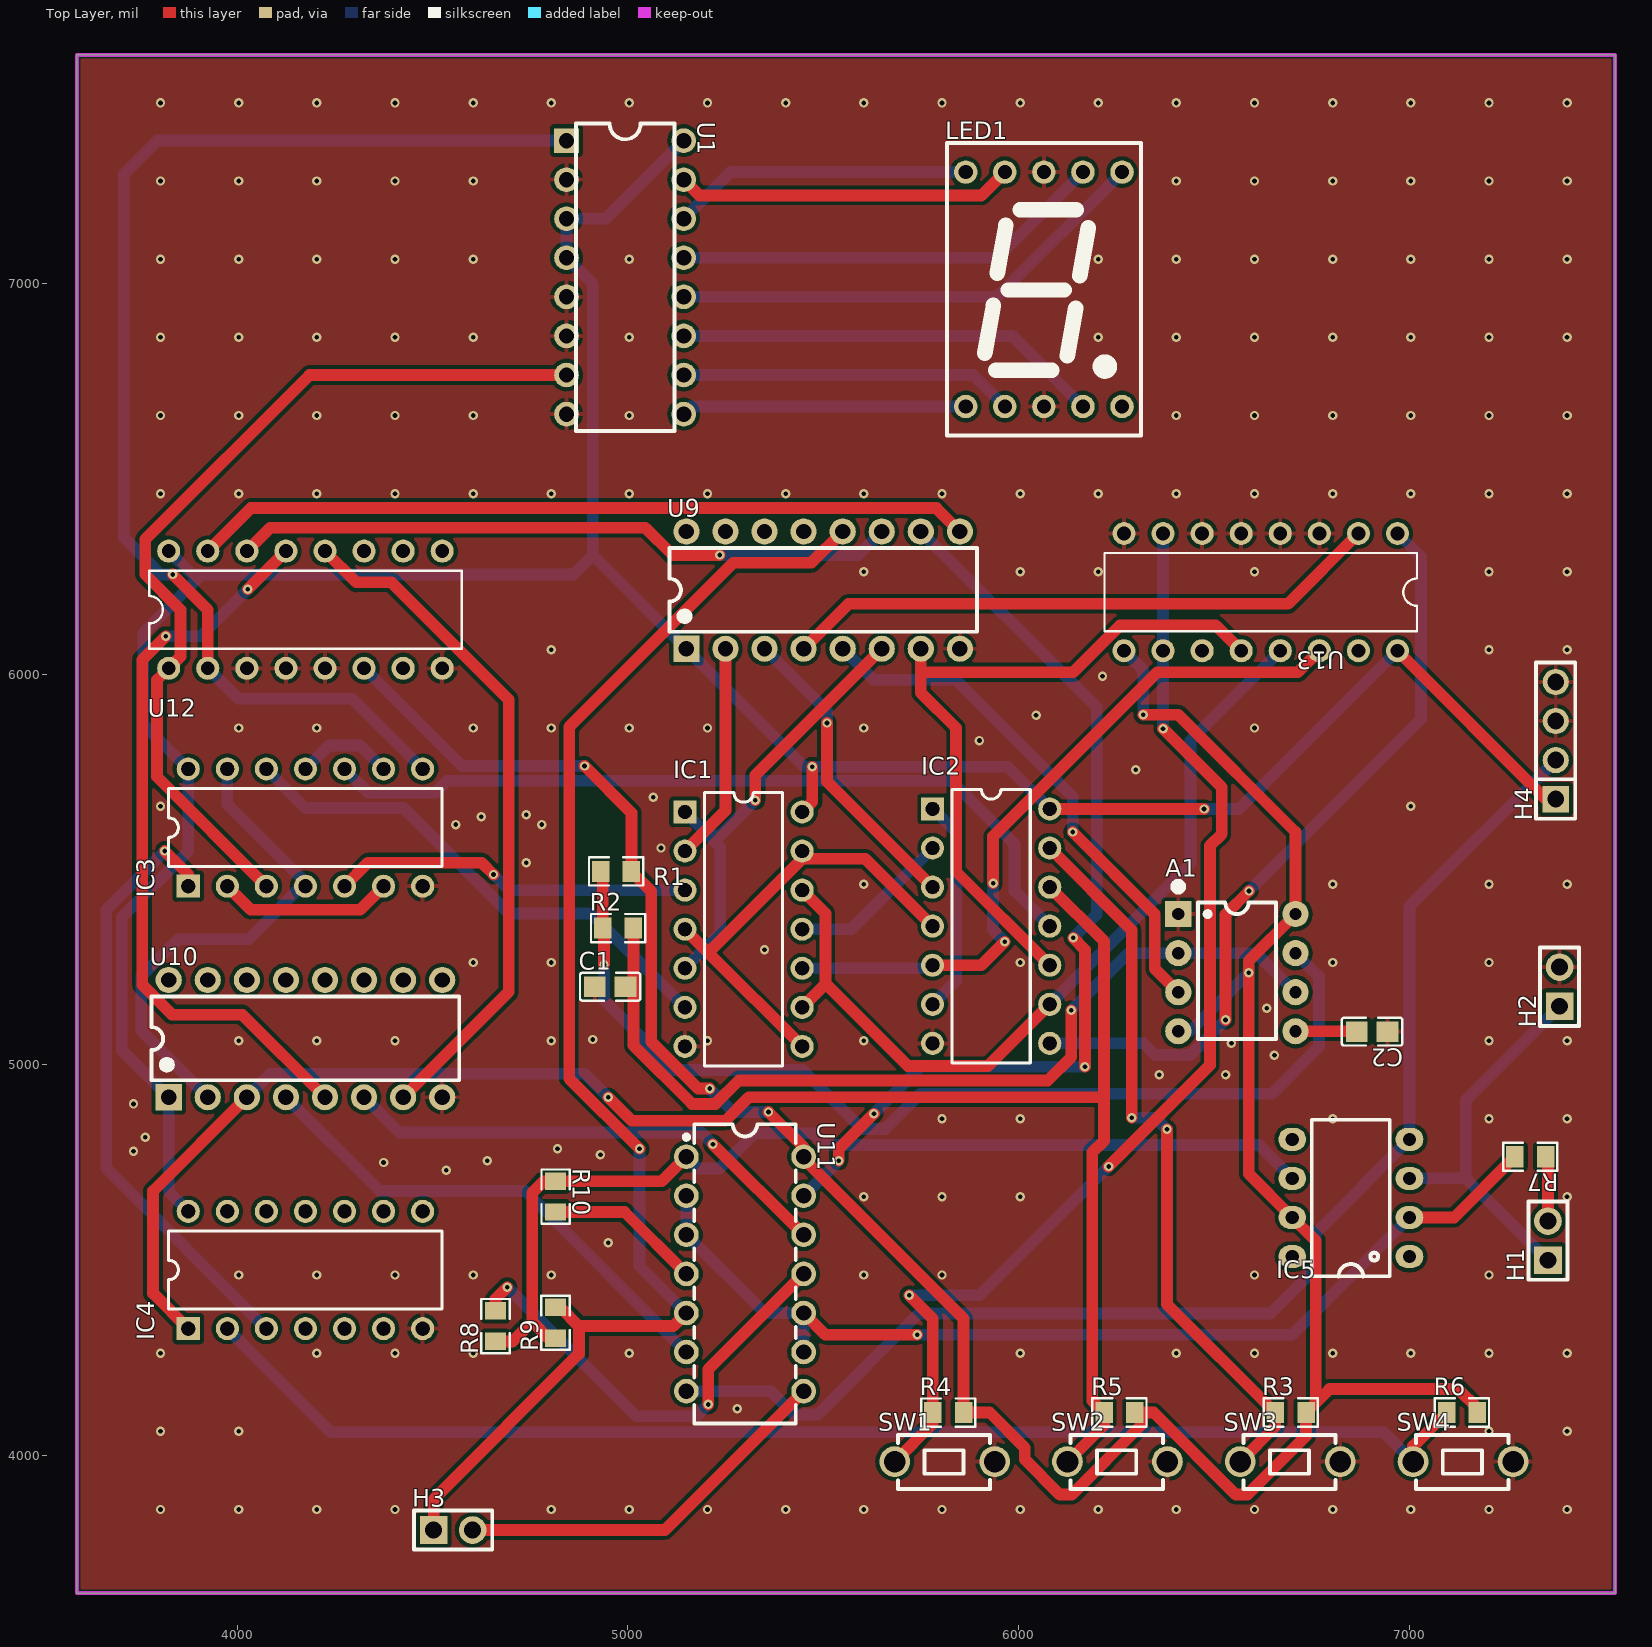
[diagram p0: Top Layer view]
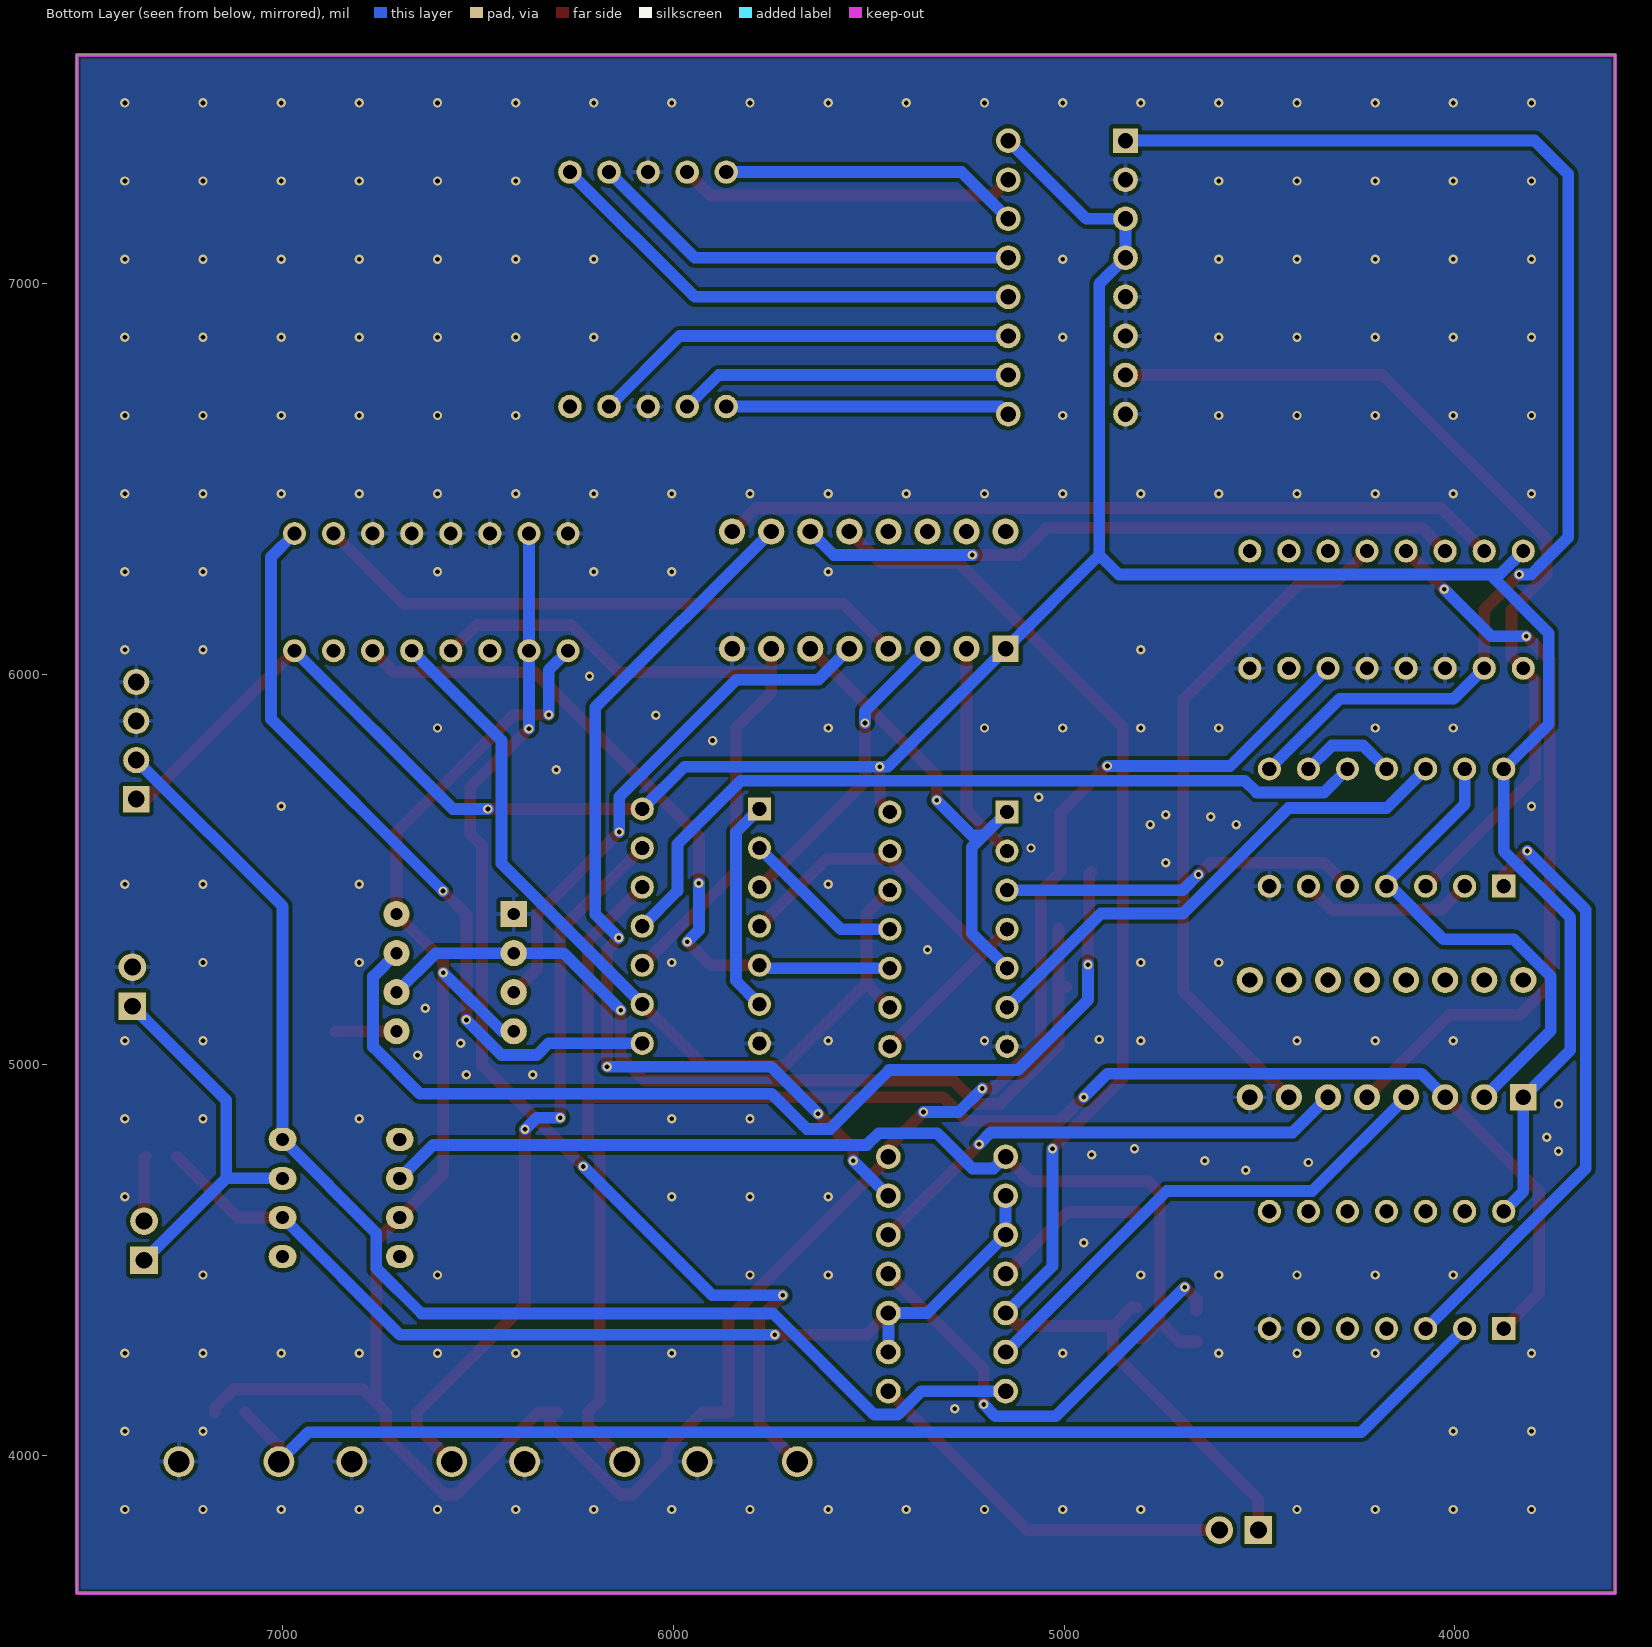
[diagram p1: Bottom Layer view, seen from below]
# Altium PCB MISC51042.pcbdoc
Units mil, origin at the board's own origin, x right, y up, seen from the top; angles counter-clockwise.
Board outline 3937.01 x 3937.01 mil, 2 copper layers (Top Layer, Bottom Layer), stack 62.206 mil thick; 33 components, 54 nets, 218 pads, 240 vias.

## Layer stack, top to bottom
Top Solder Mask Layer: solder mask 0.394, Dk 3.3
Top Layer: signal copper 1.379
Dielectric1: surface 59.449, FR4, Dk 4.5
Bottom Layer: signal copper 1.378
Bottom Solder Mask Layer: solder mask 0.394, Dk 3.3

## Board outline
3590,7585 3590,3647.99 7527.01,3647.99 7527.01,7585

## Design rules (kind name [scope] priority, off if disabled: settings)
BoardOutlineClearance copperThickness2oz_1 [All] p2 off: genericclearance=7.99 ignorepadtopadclearanceinfootprint=FALSE except(0: Arc-SplitContinuation Track-SplitContinuation SMDPad-SplitContinuation THPad-SplitContinuation Via-SplitContinuation Fill-SplitContinuation Region-SplitContinuation Poly-SplitContinuation Text-SplitContinuation Hole-SplitContinuation; 5.98: Arc-CutoutEdge SMDPad-CutoutEdge THPad-CutoutEdge Via-CutoutEdge Fill-CutoutEdge Region-CutoutEdge Text-CutoutEdge; 6.93: Hole-OutlineEdge Hole-CutoutEdge; 10: Poly-OutlineEdge Poly-CutoutEdge; 11.81: Arc-OutlineEdge Track-OutlineEdge SMDPad-OutlineEdge THPad-OutlineEdge Via-OutlineEdge Fill-OutlineEdge Region-OutlineEdge Text-OutlineEdge Track-CutoutEdge)
BoardOutlineClearance copperThickness1oz_1 [All] p4: genericclearance=4.02 ignorepadtopadclearanceinfootprint=FALSE except(0: Arc-SplitContinuation Track-SplitContinuation SMDPad-SplitContinuation THPad-SplitContinuation Via-SplitContinuation Fill-SplitContinuation Region-SplitContinuation Poly-SplitContinuation Text-SplitContinuation Hole-SplitContinuation; 6: SMDPad-CutoutEdge THPad-CutoutEdge Via-CutoutEdge Fill-CutoutEdge Region-CutoutEdge Text-CutoutEdge; 6.93: Hole-OutlineEdge Hole-CutoutEdge; 10: Poly-OutlineEdge Poly-CutoutEdge; 11.8: Arc-OutlineEdge Track-OutlineEdge SMDPad-OutlineEdge THPad-OutlineEdge Via-OutlineEdge Fill-OutlineEdge Region-OutlineEdge Text-OutlineEdge; 11.81: Arc-CutoutEdge Track-CutoutEdge)
Clearance copperThickness2oz [All] p1 off: gap=7.99 ignorepadtopadclearanceinfootprint=FALSE except(5.98: SMDPad-Track SMDPad-SMDPad THPad-Track SMDPad-THPad THPad-THPad Track-Via SMDPad-Via THPad-Via Via-Via Fill-Track Region-Track Fill-SMDPad Region-SMDPad Fill-THPad Region-THPad Fill-Via Region-Via Fill-Fill Fill-Region Region-Region Arc-Track Arc-SMDPad Arc-THPad Arc-Via Fill-Arc Region-Arc Arc-Arc Text-Track SMDPad-Text Text-THPad Text-Via Fill-Text Region-Text Arc-Text Text-Text; 6.93: Hole-Track Hole-SMDPad Hole-THPad Hole-Via Fill-Hole Region-Hole Hole-Arc Hole-Text; 10: Poly-Track Poly-SMDPad Poly-THPad Poly-Via Poly-Fill Poly-Region Poly-Poly Poly-Arc Poly-Text Poly-Hole)
Clearance copperThickness1oz [All] p3: gap=4.02 ignorepadtopadclearanceinfootprint=FALSE except(5.98: SMDPad-Track SMDPad-SMDPad THPad-Track SMDPad-THPad THPad-THPad Track-Via SMDPad-Via THPad-Via Via-Via Fill-Track Region-Track Fill-SMDPad Region-SMDPad Fill-THPad Region-THPad Fill-Via Region-Via Fill-Fill Fill-Region Region-Region; 6: Arc-Track Arc-SMDPad Arc-THPad Arc-Via Fill-Arc Region-Arc Arc-Arc Text-Track SMDPad-Text Text-THPad Text-Via Fill-Text Region-Text Arc-Text Text-Text; 6.93: Hole-Track Hole-SMDPad Hole-THPad Hole-Via Fill-Hole Region-Hole Hole-Arc Hole-Text; 10: Poly-Track Poly-SMDPad Poly-THPad Poly-Via Poly-Fill Poly-Region Poly-Poly Poly-Arc Poly-Text Poly-Hole)
Creepage creepage [All] p1: checkdistance=0 ignoreinternallayers=TRUE applytopolygonpour=TRUE
DiffPairsRouting differentialPair [All] p1: maxlimit=6 minlimit=6 mostfreqgap=6 toplayer_minwidth=5 toplayer_prefwidth=10 toplayer_maxwidth=100 toplayer_mingap=6 toplayer_prefgap=6 toplayer_maxgap=6 bottomlayer_minwidth=5 bottomlayer_prefwidth=10 bottomlayer_maxwidth=100 bottomlayer_mingap=6 bottomlayer_prefgap=6 bottomlayer_maxgap=6 maxuncoupledlength=10
HoleToHoleClearance otherClearance [All] p1: gap=11.81 allowstackedmicrovias=TRUE
Length netLength [All] p1: minlimit=0 maxlimit=0
MatchedLengths netLengthTolerance [All] p1: tolerance=1000
PasteMaskExpansion pasteMaskExpansion [All] p1: expansion=0
PlaneConnect innerPlane [All] p1: planeconnectstyle=Relief reliefexpansion=20 reliefentries=4 reliefconductorwidth=10 reliefairgap=10
PolygonConnect copperRegion [(InNet('GND'))] p1: connectstyle=Relief reliefconductorwidth=10 reliefentries=4 polygonreliefangle="90 Angle" airgapwidth=10 via.connectstyle=Relief via.reliefconductorwidth=10 via.reliefentries=4 via.polygonreliefangle="90 Angle" via.airgapwidth=10
RoutingVias viaSize [All] p1: holewidth=12.01 width=24.02 viastyle="Through Hole" minholewidth=11.81 minwidth=19.68 maxholewidth=248.03 maxwidth=393.7
SolderMaskExpansion solderMaskExpansion [IsVia] p1: expansion=-1000 istentingtop=TRUE
SolderMaskExpansion solderMaskExpansion [All] p2: expansion=2 istentingtop=FALSE
Width copperThickness2oz_2 [All] p1 off: maxlimit=100 minlimit=8 preferedwidth=10
Width copperThickness1oz_2 [All] p2: maxlimit=10 minlimit=10 preferedwidth=10 toplayer_minwidth=30 toplayer_maxwidth=100 toplayer_prefwidth=30 bottomlayer_minwidth=30 bottomlayer_maxwidth=100 bottomlayer_prefwidth=30

## Components (designator, comment, footprint, x,y, rotation, side; value= is the part's Value field where it differs from the comment)
A1 "555_VIRTUAL" 555-VIRTUAL 6559,5235.99 r0 top
C1 "10uF" C0805 4955,5200 r0 top
C2 "10nF" C0805 6905,5085 r180 top
H1 "" HDR-TH_2P-P2.54-V-M-1 7355,4550 r90 top
H2 "" HDR-TH_2P-P2.54-V-M-1 7385,5200 r90 top
H3 "" HDR-TH_2P-P2.54-V-M-1 4553.02,3809.44 r0 top
H4 "" HDR-TH_4P-P2.54-V-M 7375,5830 r90 top
IC1 "74LS00N" DIP14-300_MH 5296.32,5347.23 r0 top
IC2 "74LS00N" DIP14-300_MH 5930,5355 r0 top
IC3 "74LS00N" DIP14-300_MH 4175,5607.3 r90 top
IC4 "74LS00N" DIP14-300_MH 4175,4475 r90 top
IC5 "UA741CP" DIP8 6850.64,4659.35 r90 top
LED1 "" LED-SEG-TH_10P-L12.6-W19.0-P2.54-S15.24-BL 6065,6985 r0 top
R1 "100K" R0805 4970,5495 r180 top
R2 "20K" R0805 4975,5350 r0 top
R3 "10K" R0805 6696.67,4110.2 r0 top
R4 "10K" R0805 5820,4110 r0 top
R5 "10K" R0805 6258.33,4110.2 r0 top
R6 "10K" R0805 7135,4110.2 r0 top
R7 "10K" R0805 7310,4765 r180 top
R8 "30K" R0805 4661.38,4331.6 r90 top
R9 "20K" R0805 4815,4340 r90 top
R10 "10K" R0805 4815.12,4662.83 r270 top
SW1 "" Key_TH_3.5x6x4.3 5804.62,3984.7 r0 top
SW2 "" Key_TH_3.5x6x4.3 6246.85,3984.7 r0 top
SW3 "" Key_TH_3.5x6x4.3 6689.07,3984.7 r0 top
SW4 "" Key_TH_3.5x6x4.3 7131.29,3984.7 r0 top
U1 "" DIP-16_L19.8-W6.5-P2.54-LS7.6-BL 4993.15,7015.63 r270 top
U9 "" PDIP-16_L19.7-W6.6-P2.54-LS7.6-BL 5500,6215 r0 top
U10 "" PDIP-16_L19.7-W6.6-P2.54-LS7.6-BL 4175,5067.13 r0 top
U11 "" PDIP-14_L19.3-W6.4-P2.54-LS7.9-BL 5300,4465 r270 top
U12 "74LS138N" DIP-16_L20.32-W6.4-P2.54-LS7.6-BL 4175,6165 r0 top
U13 "74LS161DC" DIP-16_L20.32-W6.4-P2.54-LS7.6-BL 6620,6210 r180 top

## Footprints (in the part's own frame and the unit in brackets; to place one, negate y for a bottom-side part, rotate by r counter-clockwise, add the part's x,y. Pads: shape width x height; smd on the part's side, far side on the other; paste and mask are expansions set on the pad)
555-VIRTUAL [mm]
  rect 1.7x1.7 hole 0.8: 1(-3.81,3.81)
  round 1.7 hole 0.8: 2(-3.81,1.27) 3(-3.81,-1.27) 4(-3.81,-3.81) 5(3.81,-3.81) 6(3.81,-1.27) 7(3.81,1.27) 8(3.81,3.81)
  silkscreen extent -4.06,-4.32 2.54,5.84
C0805 [mm]
  rect 1.41x1.35 smd paste-100 mask+0.051: 1(-1,0) 2(1,0)
  silkscreen extent -1.96,-0.9 1.96,0.9
DIP8 [mm]
  oval 1.5x1.8 hole 0.85 paste+0 mask+0.102: 1(-3.81,-3.81) 2(-1.27,-3.81) 3(1.27,-3.81) 4(3.81,-3.81) 5(3.81,3.81) 6(1.27,3.81) 7(-1.27,3.81) 8(-3.81,3.81)
  silkscreen extent -5.1,-2.54 5.08,2.54
DIP14-300_MH [mm]
  rect 1.5x1.5 hole 0.9 slot 0.905 at 0 deg: 1(-3.81,7.62)
  round 1.5 hole 0.9 slot 0.905 at 0 deg: 2(-3.81,5.08) 3(-3.81,2.54) 4(-3.81,0) 5(-3.81,-2.54) 6(-3.81,-5.08) 7(-3.81,-7.62) 8(3.81,-7.62) 9(3.81,-5.08) 10(3.81,-2.54) 11(3.81,0) 12(3.81,2.54) 13(3.81,5.08) 14(3.81,7.62)
  silkscreen extent -2.54,-8.89 2.54,8.89
DIP-16_L19.8-W6.5-P2.54-LS7.6-BL [mm]
  rect 1.6x1.6 hole 1: 1(-8.89,-3.81)
  round 1.6 hole 1 copper offset 0,0: 2(-6.35,-3.81) 3(-3.81,-3.81) 4(-1.27,-3.81) 5(1.27,-3.81) 6(3.81,-3.81) 7(6.35,-3.81) 8(8.89,-3.81) 9(8.89,3.81) 10(6.35,3.81) 11(3.81,3.81) 12(1.27,3.81) 13(-1.27,3.81) 14(-3.81,3.81) 15(-6.35,3.81) 16(-8.89,3.81)
  silkscreen extent -10,-3.2 10,3.2
DIP-16_L20.32-W6.4-P2.54-LS7.6-BL [mm]
  round 1.5 hole 0.9: 1(-8.89,-3.81) 2(-6.35,-3.81) 3(-3.81,-3.81) 4(-1.27,-3.81) 5(1.27,-3.81) 6(3.81,-3.81) 7(6.35,-3.81) 8(8.89,-3.81) 9(8.89,3.81) 10(6.35,3.81) 11(3.81,3.81) 12(1.27,3.81) 13(-1.27,3.81) 14(-3.81,3.81) 15(-6.35,3.81) 16(-8.89,3.81)
  silkscreen extent -10.16,-2.54 10.16,2.54
HDR-TH_2P-P2.54-V-M-1 [mm]
  rect 1.8x1.8 hole 1.1: 1(-1.27,0)
  round 1.8 hole 1.1: 2(1.27,0)
  silkscreen extent -2.54,-1.27 2.54,1.27
HDR-TH_4P-P2.54-V-M [mm]
  rect 1.7x1.7 hole 1.1: 1(-3.81,0)
  round 1.7 hole 1.1: 2(-1.27,0) 3(1.27,0) 4(3.81,0)
  silkscreen extent -5.08,-1.27 5.08,1.27
Key_TH_3.5x6x4.3 [mil]
  round 78.7 hole 55.1 paste+0 mask+2: A(-121.44,0) B(134.46,0)
  silkscreen extent -114,-70 123,68
LED-SEG-TH_10P-L12.6-W19.0-P2.54-S15.24-BL [mil]
  round 60 hole 36: 1(-200,-300) 2(-100,-300) 3(0,-300) 4(100,-300) 5(200,-300) 6(200,300) 7(100,300) 8(0,300) 9(-100,300) 10(-200,300)
  silkscreen extent -248,-374 248,374
PDIP-14_L19.3-W6.4-P2.54-LS7.9-BL [mm]
  round 1.6 hole 1: 1(-7.62,-3.81) 2(-5.08,-3.81) 3(-2.54,-3.81) 4(0,-3.81) 5(2.54,-3.81) 6(5.08,-3.81) 7(7.62,-3.81) 8(7.62,3.81) 9(5.08,3.81) 10(2.54,3.81) 11(0,3.81) 12(-2.54,3.81) 13(-5.08,3.81) 14(-7.62,3.81)
  silkscreen extent -9.73,-3.96 9.73,3.3
PDIP-16_L19.7-W6.6-P2.54-LS7.6-BL [mm]
  rect 1.7x1.7 hole 1: 1(-8.89,-3.81)
  round 1.7 hole 1: 2(-6.35,-3.81) 3(-3.81,-3.81) 4(-1.27,-3.81) 5(1.27,-3.81) 6(3.81,-3.81) 7(6.35,-3.81) 8(8.89,-3.81) 9(8.89,3.81) 10(6.35,3.81) 11(3.81,3.81) 12(1.27,3.81) 13(-1.27,3.81) 14(-3.81,3.81) 15(-6.35,3.81) 16(-8.89,3.81)
  silkscreen extent -10,-2.7 10,2.73
R0805 [mm]
  rect 1.133x1.377 smd paste-100 mask+0.051: 1(-1,0) 2(1,0)
  silkscreen extent -1.76,-0.92 1.76,0.92

## Via types
v1: diameter 24.02, hole 12, Top Layer to Bottom Layer, 240 vias

## Nets (pads, with @x,y where several pads share a name; then routed paths per layer and width w, separated by ;. In a path a pad name is that pad's centre, name@x,y a point inside that pad or via, vN(x,y) a via of type N, cw(c..) or ccw(c..) an arc to the next point about the centre after c; other vN are vias at no path point)
$1N1: LED1.7 U1.13 | length 1112.7
  Bottom Layer w30: U1.13@5143.15,7065.63 5945.63,7065.63 LED1.7
$1N2: LED1.6 U1.12 | length 1254.1
  Bottom Layer w30: U1.12@5143.15,6965.63 5945.63,6965.63 LED1.6
$1N3: LED1.4 U1.11 | length 1096.7
  Bottom Layer w30: U1.11@5143.15,6865.63 5984.36,6865.63 LED1.4
$1N4: LED1.2 U1.10 | length 855.3
  Bottom Layer w30: U1.10@5143.15,6765.63 5884.36,6765.63 LED1.2
$1N5: LED1.1 U1.9 | length 729.9
  Bottom Layer w30: U1.9@5143.15,6665.63 5162.51,6685 LED1.1
$1N6: LED1.9 U1.15 | length 863.5
  Top Layer w30: U1.15@5143.15,7265.63 5183.78,7225 5905,7225 LED1.9
$1N7: LED1.10 U1.14 | length 771.3
  Bottom Layer w30: U1.14@5143.15,7165.63 5262.51,7285 LED1.10
$1N10: IC1.2 U9.2 | length 560.7
  Top Layer w30: IC1.2 5250,5650.91 U9.2
$1N11: IC1.1 IC1.5 U9.6 | length 1153.7
  Top Layer w30: v1(5326.32,5677.23) 5326.32,5741.32 U9.6
  Bottom Layer w30: IC1.5 5236.32,5337.23 5236.32,5557.23 5206.32,5587.23 ; IC1.1 5206.32,5587.23 ; v1(5326.32,5677.23) 5236.32,5587.23 5206.32,5587.23
$1N12: IC1.6 IC3.12 | length 1324
  Bottom Layer w30: IC3.12 4175.07,5657.23 4426.32,5657.23 4696.32,5387.23 4906.32,5387.23 IC1.6
$1N13: IC1.4 IC1.8 IC1.13 IC2.4 | length 1188.7
  Top Layer w30: IC1.4 5206.32,5287.23 ; IC1.8 5206.32,5287.23 ; IC1.13 IC1.13@5446.32,5527.23 ; IC2.4 5607.77,5527.23 IC1.13@5446.32,5527.23 ; 5206.32,5287.23 IC1.13@5446.32,5527.23
$1N15: IC1.10 IC2.5 U13.14 | length 1860.9
  Top Layer w30: IC2.5 5905,5255 v1(5965,5315) ; v1(5935,5465) 5935,5585 6355,6005 6715,6005 U13.14
  Bottom Layer w30: IC1.10 5772.23,5247.23 IC2.5 ; v1(5935,5465) 5935,5345 v1(5965,5315)
$1N17: IC2.3 U9.3 | length 788.1
  Top Layer w30: v1(5510,5875) 5510,5725 IC2.3
  Bottom Layer w30: U9.3 5510,5905 v1(5510,5875)
$1N18: IC1.11 IC2.2 | length 419.7
  Bottom Layer w30: IC1.11 5572.23,5347.23 IC2.2
$1N19: IC2.1 IC2.6 | length 549.7
  Bottom Layer w30: IC2.6 5840,5215 5840,5595 IC2.1
$1N20: A1.4 A1.8 IC5.7 R1.1 R3.2 R4.2 R5.2 R6.2 U11.14 U12.6 U13.9 | length 7125.6
  Top Layer w30: v1(4889.37,5765) 5009.37,5645 R1.1 5060,5444.37 5060,5059.37 5180,4939.37 v1(5210,4939.37) ; v1(5360,4879.37) 5450,4789.37 5450,4759.37 5859.37,4350 R4.2 ; R4.2@5859.57,4110.2 5926.04,4110.2 6016.04,4020.2 6016.04,3990.2 6106.04,3900.2 6136.04,3900.2 6316.04,4080.2 R5.2@6316.04,4110.2 ; R5.2 R5.2@6316.04,4110.2 ; v1(6319,5895.99) 6409,5895.99 6709,5595.99 A1.8 6589,5265.99 v1(6589,5235.99) 6589,4721 IC5.7 6760.64,4549.35 6760.64,4134.81 ; R6.2 7174.37,4121.87 7126.04,4170.2 6796.04,4170.2 6760.64,4134.81 ; R5.2@6316.04,4110.2 6346.04,4110.2 6556.04,3900.2 6586.04,3900.2 6736.04,4050.2 R3.2 6760.64,4134.81
  Bottom Layer w30: U12.6 4575,5765 v1(4889.37,5765) ; v1(5210,4939.37) 5270,4879.37 v1(5360,4879.37) ; U13.9 6319,6011 v1(6319,5895.99) ; A1.4 6439,5085.99 v1(6589,5235.99)
$1N21: A1.7 R1.2 R2.1 | length 2650.6
  Top Layer w30: R1.2 4935.63,5490 R2.1 4939,5346.63 v1(4939,5256.63)
  Bottom Layer w30: v1(4939,5256.63) 4939,5166.63 5119,4986.63 5448.37,4986.63 5599,4836 5659,4836 5749,4926 6649,4926 6769,5045.99 6769,5225.99 A1.7
$1N22: A1.2 A1.6 C1.2 R2.2 | length 2348.4
  Top Layer w30: C1.2 C1.2@5014.37,5200 ; R2.2 C1.2@5014.37,5200 ; v1(6134.99,5140) 6134.99,5020 6074.99,4960 5284.37,4960 5224.37,4900 5164.37,4900 5014.37,5050 C1.2@5014.37,5200
  Bottom Layer w30: v1(6134.99,5140) 6280.99,5285.99 A1.2 6609,5285.99 A1.6
$1N24: A1.5 C2.2 | length 157
  Top Layer w30: A1.5 6864.63,5085.99 C2.2
$1N25: A1.3 U9.5 | length 1357.8
  Top Layer w30: v1(6139,5596) 6349,5386 6349,5245.99 A1.3
  Bottom Layer w30: U9.5 5629,5986 5839,5986 6139,5686 v1(6139,5596)
$1N26: U9.4 U13.2 | length 1542.2
  Top Layer w30: U9.4 5565,6180 6690,6180 U13.2
$1N30: R4.1 SW1.A U13.7 U13.10 | length 2939.2
  Top Layer w30: SW1.A 5780.63,4082.15 R4.1 5780.63,4350 v1(5720.63,4410) ; v1(6230.63,4740) 6490,4999.37 6490,5560.62 6520,5590.62 6520,5710.62 v1(6370,5860.62)
  Bottom Layer w30: v1(5720.63,4410) 5900.63,4410 v1(6230.63,4740) ; v1(6370,5860.62) U13.10 U13.7
$1N31: IC2.8 U13.1 | length 1976.7
  Top Layer w30: v1(6530,5115) 6530,5385 v1(6590,5445)
  Bottom Layer w30: IC2.8 6320,5055 6350,5025 6440,5025 v1(6530,5115) ; v1(6590,5445) 7030,5885 7030,6300 U13.1
$1N32: IC2.10 U9.7 U13.12 | length 1843.3
  Top Layer w30: U9.7 5750,6005 ; IC2.10 5840,5495 5840,5862.48 5750,5952.48 5750,6005 ; U13.12 6505.01,6125 6260,6125 6140,6005 5750,6005
$1N33: IC1.9 IC1.12 IC2.9 U13.13 | length 2225.1
  Top Layer w30: IC1.9 5506.32,5207.23 ; IC1.12 5506.32,5387.23 5506.32,5207.23 ; IC2.9 5922.23,4997.23 5716.32,4997.23 5506.32,5207.23
  Bottom Layer w30: IC2.9 6440,5515 6440,5830 U13.13
$1N35: IC5.6 R8.1 R9.1 R10.1 U11.1 | length 2603.1
  Top Layer w30: R8.1 4705.14,4292.22 4755.12,4342.2 ; R9.1 4796.7,4300.63 4755.12,4342.2 ; U11.1 5087.2,4702.2 R10.1 4785.12,4702.2 4755.12,4672.2 4755.12,4342.2
  Bottom Layer w30: U11.1 5180,4735 5235,4735 5325,4825 5475,4825 5505,4795 6615,4795 IC5.6
$1N36: IC5.2 R7.2 U11.2 U11.3 U11.9 U11.10 | length 2615.3
  Top Layer w30: U11.10 5505.65,4309.35 v1(5740.64,4309.35) ; IC5.2 7114.98,4609.35 R7.2
  Bottom Layer w30: U11.2 U11.3 5350,4365 U11.10 U11.9 ; v1(5740.64,4309.35) 6700.64,4309.35 IC5.2
$1N37: H1.2 R7.1 | length 167.3
  Top Layer w30: R7.1 7355,4759.37 H1.2
$1N38: H1.1 H2.1 IC5.3 | length 981
  Bottom Layer w30: IC5.3 7001.29,4710 7145,4710 ; H1.1 7145,4710 ; H2.1 7145,4910 7145,4710
$1N39: U9.9 U12.15 | length 1995.4
  Top Layer w30: U12.15 4035,6425 5790,6425 U9.9
$1N40: U9.11 U12.14 | length 1703.7
  Top Layer w30: U12.14 4085,6375 5045,6375 5115,6305 v1(5235,6305)
  Bottom Layer w30: v1(5235,6305) 5590,6305 U9.11
$1N41: U10.5 U12.13 | length 1902.2
  Top Layer w30: v1(3817.13,6097.13) 3757.13,6037.13 3757.13,5205 3833.64,5128.49 4013.64,5128.49 U10.5 ; v1(4027.13,6217.13) U12.13
  Bottom Layer w30: v1(3817.13,6097.13) 3907.13,6097.13 v1(4027.13,6217.13)
$1N42: U10.7 U12.12 | length 1757.1
  Top Layer w30: U12.12 4305,6235 4395,6235 4695,5935 4695,5187.13 U10.7
$1N43: U9.10 U11.13 | length 2467.9
  Top Layer w30: v1(5540,4755) 5540,4785 v1(5630,4875) ; v1(6140,5325) 6170,5295 v1(6170,4995)
  Bottom Layer w30: U11.13 v1(5540,4755) ; v1(5630,4875) 5750,4995 v1(6170,4995) ; U9.10 6200,5915 6200,5385 v1(6140,5325)
$1N44: H3.1 R9.2 U9.12 U11.5 | length 3576.2
  Top Layer w30: H3.1 4503.02,3888.18 4875,4260.16 4875,4331.42 ; R9.2 4827.05,4379.37 4875,4331.42 ; v1(5030,4785) 4850,4965 4850,5865 5270,6285 5470,6285 U9.12 ; U11.5 5116.42,4331.42 4875,4331.42
  Bottom Layer w30: v1(5030,4785) 5030,4485 U11.5
$1N45: U10.4 U11.6 | length 1295.1
  Bottom Layer w30: U10.4 4365,4677.13 4737.87,4677.13 U11.6
$1N46: U10.6 U11.12 | length 1270.9
  Top Layer w30: v1(5217.87,4797.13) U11.12
  Bottom Layer w30: U10.6 4415,4827.13 5187.87,4827.13 v1(5217.87,4797.13)
$1N47: R8.2 U11.11 | length 1171.2
  Top Layer w30: R8.2 4661.38,4400.96 v1(4691.38,4430.96) ; v1(5205.96,4130.97) 5205.96,4220.97 U11.11
  Bottom Layer w30: v1(4691.38,4430.96) 5021.38,4100.97 5175.96,4100.97 v1(5205.96,4130.97)
$1N48: R10.2 U11.4 | length 400.5
  Top Layer w30: R10.2 4991.54,4623.46 U11.4
$1N49: H3.2 U11.8 | length 994.3
  Top Layer w30: H3.2 5094.44,3809.44 U11.8
$1N64: IC1.3 IC3.5 | length 925.2
  Top Layer w30: IC3.5 4335,5517.3 4626.25,5517.3 v1(4656.25,5487.3)
  Bottom Layer w30: v1(4656.25,5487.3) 4696.32,5447.23 IC1.3
$1N65: IC3.4 IC3.13 U10.2 | length 1282.8
  Bottom Layer w30: U10.2 3755,5087.13 3755,5227.3 3849.32,5321.62 4029.32,5321.62 IC3.4@4175,5467.3 ; IC3.13 3975,5667.3 IC3.4@4175,5467.3 ; IC3.4 IC3.4@4175,5467.3
$1N66: IC2.12 IC4.1 R5.1 SW2.A U10.3 | length 4617.3
  Top Layer w30: IC4.1 3785,4415 3785,4677.13 U10.3 ; v1(4950.06,4917.13) 5010.06,4857.13 5250.06,4857.13 5310.06,4917.13 6210.06,4917.13 6218.96,4926.03 ; IC2.12 6218.96,5316.03 6218.96,4926.03 ; SW2.A 6218.96,4078.26 R5.1 6188.96,4140.2 6188.96,4776.03 6218.96,4806.03 6218.96,4926.03
  Bottom Layer w30: U10.3 4085,4977.13 4890.06,4977.13 v1(4950.06,4917.13)
$1N67: IC4.2 R6.1 SW4.A | length 3336.8
  Top Layer w30: SW4.A 7009.85,4024.43 R6.1
  Bottom Layer w30: IC4.2 4240,4060 6934.56,4060 SW4.A
$1N68: IC3.9 IC3.11 | length 249.7
  Bottom Layer w30: IC3.11 4235,5817.3 4315,5817.3 IC3.9
$1N69: IC2.11 IC3.10 | length 2066.8
  Bottom Layer w30: IC3.10 4335,5697.3 4507.7,5697.3 4537.7,5727.3 5827.7,5727.3 5990,5565 5990,5445 IC2.11
$1N70: IC2.13 R3.1 SW3.A | length 1881.7
  Top Layer w30: IC2.13 6290,5345 v1(6290,4865) ; v1(6380,4835) 6380,4387.5 R3.1 6657.3,4074.37 SW3.A
  Bottom Layer w30: v1(6290,4865) 6350,4865 v1(6380,4835)
$1N71: IC3.2 IC3.6 | length 449.7
  Top Layer w30: IC3.2 4035,5397.3 4315,5397.3 IC3.6
$1N72: IC3.1 IC4.3 | length 1569.1
  Top Layer w30: v1(3815,5547.3) 3875,5487.3 IC3.1
  Bottom Layer w30: v1(3815,5547.3) 3665,5397.3 3665,4735 IC4.3
$1N73: IC3.3 U1.7 U12.1 | length 2318.2
  Top Layer w30: IC3.3 3795,5737.3 3795,5985 U12.1 3855,6045 3855,6165 3765,6255 3765,6345 4185.63,6765.63 U1.7@4843.15,6765.63
$1N74: IC3.8 U1.1 U12.2 | length 3197
  Top Layer w30: v1(3835,6255) 3925,6165 U12.2
  Bottom Layer w30: v1(3835,6255) 3805,6255 3770.24,6289.76 3710,6350 3710,7280 3795.63,7365.63 U1.1 ; U12.2 4002.7,5937.3 4295,5937.3 IC3.8
GND: A1.1 C1.1 C2.1 H2.2 H4.3 H4.4 IC1.7 IC2.7 IC3.7 IC4.7 LED1.3 LED1.8 SW1.B SW2.B SW3.B SW4.B U1.2 U1.5 U1.6 U1.8 U9.8 U10.8 U12.3 U12.4 U12.5 U12.8 U13.3 U13.4 U13.5 U13.6 U13.8
  other v1: 3804.1,3862.09 4004.1,3862.09 4204.1,3862.09 4404.1,3862.09 4804.1,3862.09 5004.1,3862.09 5204.1,3862.09 5404.1,3862.09 5604.1,3862.09 5804.1,3862.09 6004.1,3862.09 6204.1,3862.09 6404.1,3862.09 6604.1,3862.09 6804.1,3862.09 7004.1,3862.09 7204.1,3862.09 7404.1,3862.09 3804.1,4062.09 4004.1,4062.09 7204.1,4062.09 7404.1,4062.09 5280,4120 3804.1,4262.09 4204.1,4262.09 4404.1,4262.09 4604.1,4262.09 5004.1,4262.09 6004.1,4262.09 6404.1,4262.09 6604.1,4262.09 6804.1,4262.09 7004.1,4262.09 7204.1,4262.09 7404.1,4262.09 4004.1,4462.09 4204.1,4462.09 4404.1,4462.09 4604.1,4462.09 4804.1,4462.09 5604.1,4462.09 5804.1,4462.09 6604.1,4462.09 7204.1,4462.09 4950,4545 5604.1,4662.09 5804.1,4662.09 6004.1,4662.09 7404.1,4662.09 4535,4730 4375,4750 4640,4755 4930,4770 3735,4778.74 4820,4785 3765,4815 5804.1,4862.09 6004.1,4862.09 6804.1,4862.09 7204.1,4862.09 7404.1,4862.09 3735,4900 6360,4975 6530,4975 6655,5025 6545,5055 4004.1,5062.09 4204.1,5062.09 4404.1,5062.09 4804.1,5062.09 5204.1,5062.09 5604.1,5062.09 7204.1,5062.09 7404.1,5062.09 4910,5065 6635,5145 4604.1,5262.09 4804.1,5262.09 6004.1,5262.09 6804.1,5262.09 7204.1,5262.09 5350,5295 5604.1,5462.09 6804.1,5462.09 7204.1,5462.09 7404.1,5462.09 4740,5516.96 5085,5555 4560,5615 4780,5615 4625,5635 4740,5640 3804.1,5662.09 7004.1,5662.09 5065,5685 6300,5755 5900,5830 4004.1,5862.09 4204.1,5862.09 4604.1,5862.09 4804.1,5862.09 5004.1,5862.09 5204.1,5862.09 5604.1,5862.09 6604.1,5862.09 6045,5895 6215,5995 4804.1,6062.09 7204.1,6062.09 7404.1,6062.09 5604.1,6262.09 6004.1,6262.09 6204.1,6262.09 6604.1,6262.09 7204.1,6262.09 7404.1,6262.09 3804.1,6462.09 4004.1,6462.09 4204.1,6462.09 4404.1,6462.09 4604.1,6462.09 4804.1,6462.09 5004.1,6462.09 5204.1,6462.09 5404.1,6462.09 5604.1,6462.09 5804.1,6462.09 6004.1,6462.09 6204.1,6462.09 6404.1,6462.09 6604.1,6462.09 6804.1,6462.09 7004.1,6462.09 7204.1,6462.09 7404.1,6462.09 3804.1,6662.09 4004.1,6662.09 4204.1,6662.09 4404.1,6662.09 4604.1,6662.09 5004.1,6662.09 6404.1,6662.09 6604.1,6662.09 6804.1,6662.09 7004.1,6662.09 7204.1,6662.09 7404.1,6662.09 3804.1,6862.09 4004.1,6862.09 4204.1,6862.09 4404.1,6862.09 4604.1,6862.09 5004.1,6862.09 6204.1,6862.09 6404.1,6862.09 6604.1,6862.09 6804.1,6862.09 7004.1,6862.09 7204.1,6862.09 7404.1,6862.09 3804.1,7062.09 4004.1,7062.09 4204.1,7062.09 4404.1,7062.09 4604.1,7062.09 5004.1,7062.09 6204.1,7062.09 6404.1,7062.09 6604.1,7062.09 6804.1,7062.09 7004.1,7062.09 7204.1,7062.09 7404.1,7062.09 3804.1,7262.09 4004.1,7262.09 4204.1,7262.09 4404.1,7262.09 4604.1,7262.09 6404.1,7262.09 6604.1,7262.09 6804.1,7262.09 7004.1,7262.09 7204.1,7262.09 7404.1,7262.09 3804.1,7462.09 4004.1,7462.09 4204.1,7462.09 4404.1,7462.09 4604.1,7462.09 4804.1,7462.09 5004.1,7462.09 5204.1,7462.09 5404.1,7462.09 5604.1,7462.09 5804.1,7462.09 6004.1,7462.09 6204.1,7462.09 6404.1,7462.09 6604.1,7462.09 6804.1,7462.09 7004.1,7462.09 7204.1,7462.09 7404.1,7462.09
VCC: H4.1 IC1.14 IC2.14 IC3.14 IC4.14 U1.3 U1.4 U1.16 U9.1 U10.1 U12.16 U13.16 | length 7468.4
  Top Layer w30: IC1.14 5472.23,5673.14 v1(5472.23,5763.14) ; IC2.14 v1(6475,5655) ; U13.16 7350,5680 H4.1
  Bottom Layer w30: U12.16 3885,6255 3910,6255 ; IC4.14 3825,4675 U10.1 3705,5037.13 3705,5377.3 3875,5547.3 IC3.14 3760,5872.3 3760,6105 3910,6255 ; U1.16@5143.15,7365.63 4943.15,7165.63 4843.15,7165.63 4843.15,7065.63 4910,6998.78 4910,6305 ; IC2.14 5971.86,5763.14 v1(5472.23,5763.14) 5451.87,5763.14 U9.1 4910,6305 ; v1(6475,5655) 6565,5655 U13.16 ; 3910,6255 4860,6255 4910,6305
VEE: H4.2 IC5.4 U11.7 | length 3345.7
  Bottom Layer w30: U11.7 5366.29,4165 5426.29,4105 5486.29,4105 5744.97,4363.68 6644.97,4363.68 6760.64,4479.35 6760.64,4569.35 IC5.4 7000.64,5405.64 H4.2
pads on no net: IC4.4 IC4.5 IC4.6 IC4.8 IC4.9 IC4.10 IC4.11 IC4.12 IC4.13 IC5.1 IC5.5 IC5.8 LED1.5 U9.13 U9.14 U9.15 U9.16 U10.9 U10.10 U10.11 U10.12 U10.13 U10.14 U10.15 U10.16 U12.7 U12.9 U12.10 U12.11 U13.11 U13.15

## Polygon pours and split planes (outlines as drawn)
GND on Top Layer (solid, remove dead copper, pour order 0): 3035,8100 3035,3000 8355,3000 8355,8100
GND on Bottom Layer (solid, remove dead copper, pour order 2): 3000,7985 3000,3455 7700,3455 7700,7985

## Keep-outs
Board Outline Layer:
  the board outline again, w10